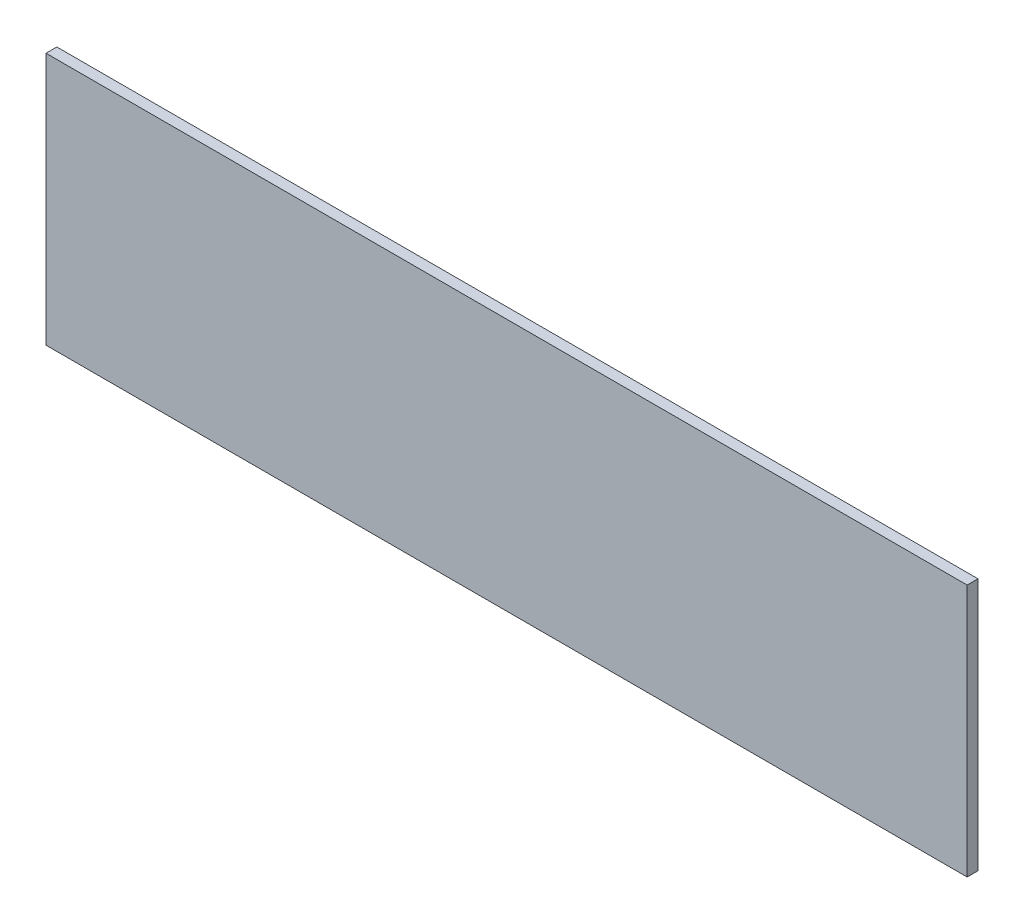
from build123d import *

# Parameters (mm, degrees)
SKETCH_1_W      = 255
SKETCH_1_H      = 70
EXTRUDE_1_DEPTH = 3


with BuildPart() as part:
    # 草图1 → 凸台-拉伸1 (new body)
    with BuildSketch(Plane.XY):
        with Locations((127.5, 35)):
            Rectangle(SKETCH_1_W, SKETCH_1_H)
    extrude(amount=EXTRUDE_1_DEPTH)


solid = part.part
